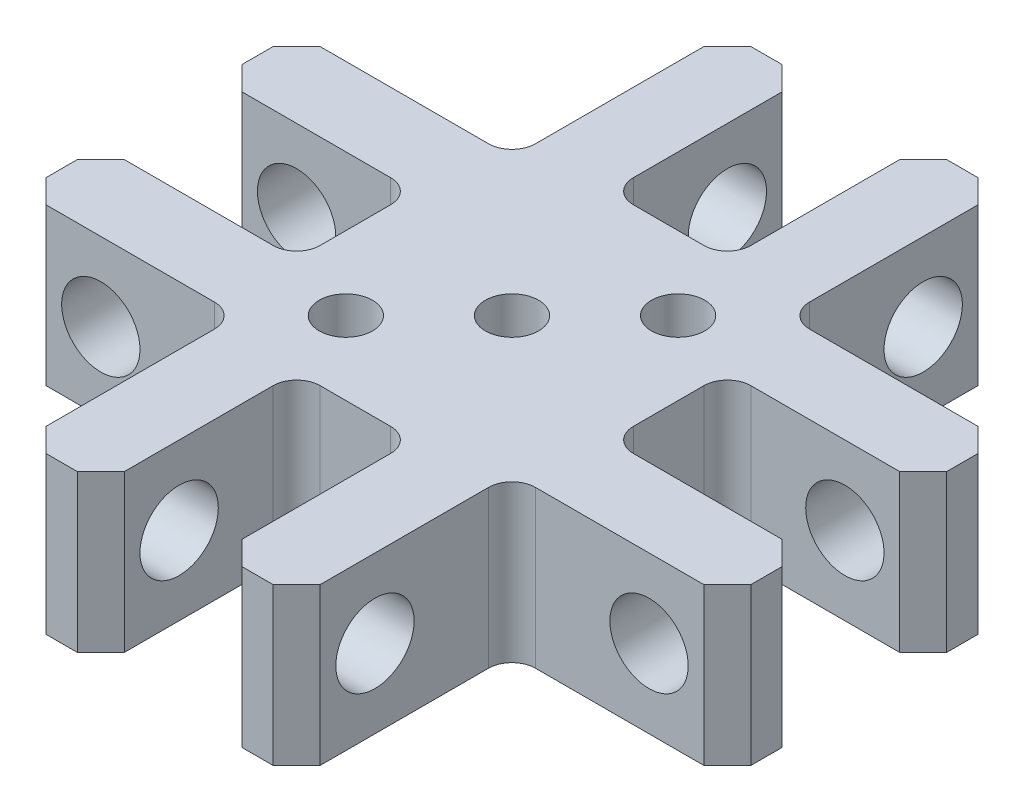
SolidWorks part; units mm, degrees
ref_plane "Front Plane" through (0, 0, 0) normal (0, 0, 1) x (1, 0, 0)
ref_plane "Top Plane" through (0, 0, 0) normal (0, 1, 0) x (1, 0, 0)
ref_plane "Right Plane" through (0, 0, 0) normal (1, 0, 0) x (0, 0, -1)
other "Configuration Table"
sketch "Sketch1" plane through (0, 0, 0) normal (0, 1, 0) x (1, 0, 0)
  line L8 (-45, 45) -> (45, 45)
  line L9 (-45, 45) -> (-45, -45)
  line L10 (-45, -45) -> (45, -45)
  line L11 (45, 45) -> (45, -45)
  line L12 (-45, 45) -> (45, -45) construction
  line L13 (-45, -45) -> (45, 45) construction
  point P0 (0, 0)
  dimension "D1" = 90
  dimension "D2" = 90
extrude "Boss-Extrude1" add sketch "Sketch1" along normal blind 20 contours L10 L11 L8 L9
chamfer "Chamfer1" distance 3 angle 45 4 edges at (-45, 10, 45) (45, 10, 45) (45, 10, -45) (-45, 10, -45)
hole_wizard "M8 Tapped Hole1" positions "Sketch2" profile "Sketch3" tap size "M8" standard "GB"
sketch "Sketch2" plane through (0, 20, 0) normal (0, 1, 0) x (1, 0, 0)
  point P0 (0, 0)
sketch "Sketch3" plane through (0, 20, 0) normal (1, 0, 0) x (0, 0, 1)
  line L0 (0, 0) -> (0, 21.7929)
  line L1 (0, 21.7929) -> (3.4, 19.75)
  line L2 (3.4, 19.75) -> (3.4, 0)
  line L5 (3.4, 0) -> (0, 0)
  line L10 (0, 21.7929) -> (-3.4, 19.75) construction
  line L11 (0, -6.35) -> (0, 107.95) construction
  dimension "螺纹孔钻头直径" = 6.8
  dimension "螺纹孔钻头深度" = 19.75
  dimension "导头角度" = 118
cosmetic thread "Cosmetic Thread1" parameters "D1"=16, "D2"=8
sketch "Sketch4" plane through (0, 20, 0) normal (0, 1, 0) x (1, 0, 0)
  line L0 (-42, 45) -> (42, 45) construction
  line L1 (-7.5, 45) -> (7.5, 45)
  line L2 (-7.5, 45) -> (-7.5, 20)
  line L3 (-7.5, 20) -> (7.5, 20)
  line L4 (7.5, 45) -> (7.5, 20)
  line L5 (-7.5, 45) -> (7.5, 20) construction
  line L6 (-7.5, 20) -> (7.5, 45) construction
  point P0 (0, 32.5)
  dimension "D1" = 25
  dimension "D2" = 15
extrude "Cut-Extrude1" cut sketch "Sketch4" against normal blind 42
fillet "Fillet1" radius 3 2 edges at (7.5, 10, -20) (-7.5, 10, -20)
chamfer "Chamfer2" distance 3 angle 45 2 edges at (7.5, 10, -45) (-7.5, 10, -45)
pattern_circular "CirPattern2" count 4 every 90 about axis through (0, 0, 0) along (0, 1, 0) of "Cut-Extrude1", "Fillet1"
chamfer "Chamfer3" distance 3 angle 45 6 edges at (-45, 10, -7.5) (-45, 10, 7.5) (45, 10, -7.5) (45, 10, 7.5) (7.5, 10, 45) (-7.5, 10, 45)
sketch "Sketch5" plane through (0, 20, 0) normal (0, 1, 0) x (1, 0, 0)
  line L0 (-7.5, 42) -> (-7.5, 23) construction
  line L1 (-45, 45) -> (-17.5, 45)
  line L2 (-45, 45) -> (-45, 17.5)
  line L3 (-45, 17.5) -> (-17.5, 17.5)
  line L4 (-17.5, 45) -> (-17.5, 17.5)
  line L5 (-45, 42) -> (-45, 10.5) construction
  line L6 (-42, 45) -> (-10.5, 45) construction
  line L7 (-23, 7.5) -> (-42, 7.5) construction
  dimension "D1" = 10
  dimension "D2" = 10
extrude "Cut-Extrude2" cut sketch "Sketch5" against normal blind 42
pattern_circular "CirPattern3" count 4 every 90 about axis through (0, 0, 0) along (0, 1, 0) of "Cut-Extrude2"
chamfer "Chamfer4" distance 3 angle 45 8 edges at (17.5, 10, -45) (45, 10, -17.5) (17.5, 10, 45) (45, 10, 17.5) (-17.5, 10, 45) (-45, 10, 17.5) (-45, 10, -17.5) (-17.5, 10, -45)
fillet "Fillet2" radius 3 4 edges at (-17.5, 10, 17.5) (17.5, 10, 17.5) (17.5, 10, -17.5) (-17.5, 10, -17.5)
sketch "Sketch6" plane through (-17.5, 0, 0) normal (-1, 0, 0) x (0, 0, 1)
  line L0 (-20.5, 20) -> (-42, 20) construction
  line L1 (-45, 0) -> (-45, 20) construction
  circle A0 centre (-35, 10) radius 5
  dimension "D1" = 10
  dimension "D2" = 10
  dimension "D3" = 10
extrude "Cut-Extrude3" cut sketch "Sketch6" against normal blind 42
pattern_circular "CirPattern4" count 4 every 90 about axis through (0, 20, 0) along (0, 1, 0) of "Cut-Extrude3"
hole_wizard "M8 Tapped Hole2" positions "Sketch8" profile "Sketch9" tap size "M8" standard "GB"
sketch "Sketch8" plane through (0, 20, 0) normal (0, 1, 0) x (1, 0, 0)
  line L0 (18.3787, 18.3787) -> (-18.3787, -18.3787) construction
  arc A0 (17.5, 20.5) -> (20.5, 17.5) centre (20.5, 20.5) ccw construction
  arc A1 (-17.5, -20.5) -> (-20.5, -17.5) centre (-20.5, -20.5) ccw construction
  point P11 (10.6066, 10.6066)
  point P13 (-10.6066, -10.6066)
  dimension "D1" = 15
  dimension "D2" = 15
sketch "Sketch9" plane through (-10.6066, 20, 10.6066) normal (1, 0, 0) x (0, 0, 1)
  line L0 (0, 0) -> (0, 21.7929)
  line L1 (0, 21.7929) -> (3.4, 19.75)
  line L2 (3.4, 19.75) -> (3.4, 0)
  line L5 (3.4, 0) -> (0, 0)
  line L10 (0, 21.7929) -> (-3.4, 19.75) construction
  line L11 (0, -6.35) -> (0, 107.95) construction
  dimension "螺纹孔钻头直径" = 6.8
  dimension "螺纹孔钻头深度" = 19.75
  dimension "导头角度" = 118
cosmetic thread "Cosmetic Thread2" parameters "D1"=16, "D2"=8
cosmetic thread "Cosmetic Thread3" parameters "D1"=16, "D2"=8
